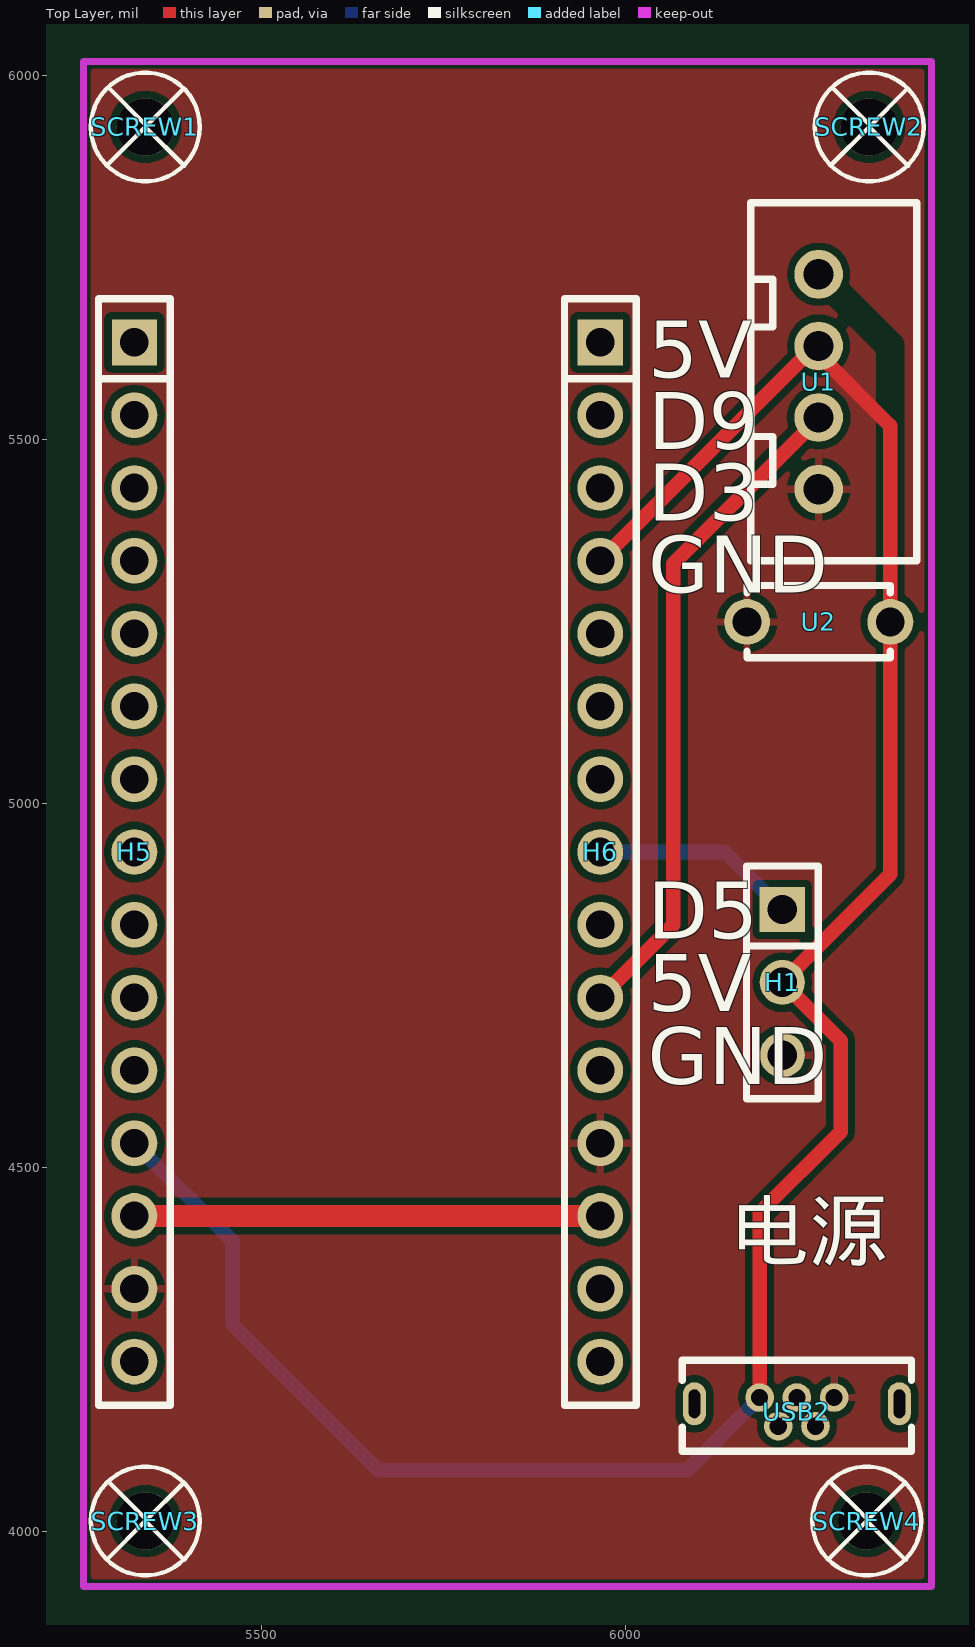
[diagram p0: Top Layer view]
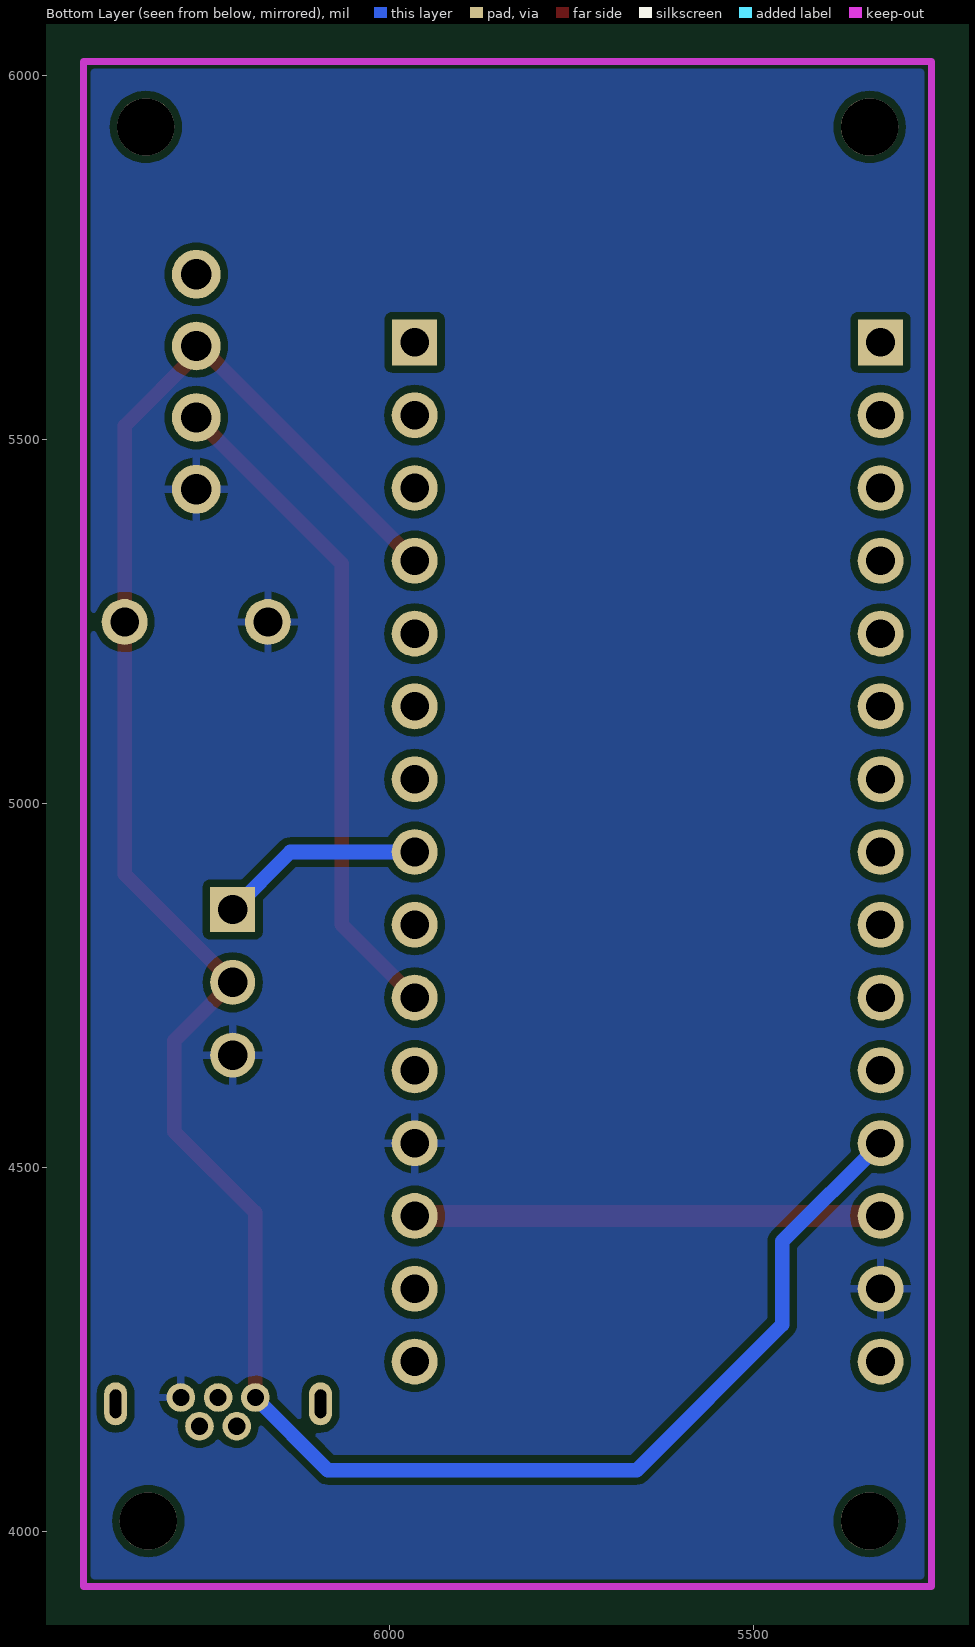
[diagram p1: Bottom Layer view, seen from below]
# Altium PCB MISC52018.pcbdoc
Units mil, origin at the board's own origin, x right, y up, seen from the top; angles counter-clockwise.
Board outline 5430 x 4915 mil, 2 copper layers (Top Layer, Bottom Layer), stack 62.206 mil thick; 10 components, 26 nets, 50 pads, 0 vias.

## Layer stack, top to bottom
Top Solder Mask Layer: solder mask 0.394, Dk 3.3
Top Layer: signal copper 1.379
Dielectric1: surface 59.449, FR4, Dk 4.5
Bottom Layer: signal copper 1.378
Bottom Solder Mask Layer: solder mask 0.394, Dk 3.3

## Board outline
8180,2750 2750,2750 2750,7665 8180,7665

## Design rules (kind name [scope] priority, off if disabled: settings)
BoardOutlineClearance copperThickness2oz_1 [All] p2 off: genericclearance=7.99 ignorepadtopadclearanceinfootprint=FALSE except(0: Arc-SplitContinuation Track-SplitContinuation SMDPad-SplitContinuation THPad-SplitContinuation Via-SplitContinuation Fill-SplitContinuation Region-SplitContinuation Poly-SplitContinuation Text-SplitContinuation Hole-SplitContinuation; 5.98: Arc-CutoutEdge Track-CutoutEdge SMDPad-CutoutEdge THPad-CutoutEdge Via-CutoutEdge Text-CutoutEdge; 6.9: Hole-OutlineEdge Hole-CutoutEdge; 10: Poly-OutlineEdge Poly-CutoutEdge; 11.81: Arc-OutlineEdge Track-OutlineEdge SMDPad-OutlineEdge THPad-OutlineEdge Via-OutlineEdge Fill-OutlineEdge Region-OutlineEdge Text-OutlineEdge Fill-CutoutEdge Region-CutoutEdge)
BoardOutlineClearance Plane_innerPlane_1 [All] p4 off: genericclearance=4.02 ignorepadtopadclearanceinfootprint=FALSE except(0: Arc-SplitContinuation Track-SplitContinuation SMDPad-SplitContinuation THPad-SplitContinuation Via-SplitContinuation Fill-SplitContinuation Region-SplitContinuation Poly-SplitContinuation Text-SplitContinuation Hole-SplitContinuation; 5.98: Arc-CutoutEdge Track-CutoutEdge SMDPad-CutoutEdge THPad-CutoutEdge Via-CutoutEdge Text-CutoutEdge; 6.9: Hole-OutlineEdge Hole-CutoutEdge; 10: Poly-OutlineEdge Poly-CutoutEdge; 11.81: Arc-OutlineEdge Track-OutlineEdge SMDPad-OutlineEdge THPad-OutlineEdge Via-OutlineEdge Fill-OutlineEdge Region-OutlineEdge Text-OutlineEdge Fill-CutoutEdge Region-CutoutEdge)
BoardOutlineClearance Copper_copperRegion_1 [All] p6 off: genericclearance=4.02 ignorepadtopadclearanceinfootprint=FALSE except(0: Arc-SplitContinuation Track-SplitContinuation SMDPad-SplitContinuation THPad-SplitContinuation Via-SplitContinuation Fill-SplitContinuation Region-SplitContinuation Poly-SplitContinuation Text-SplitContinuation Hole-SplitContinuation; 5.98: Arc-CutoutEdge Track-CutoutEdge SMDPad-CutoutEdge THPad-CutoutEdge Via-CutoutEdge Text-CutoutEdge; 6.9: Hole-OutlineEdge Hole-CutoutEdge; 10: Poly-OutlineEdge Poly-CutoutEdge; 11.81: Arc-OutlineEdge Track-OutlineEdge SMDPad-OutlineEdge THPad-OutlineEdge Via-OutlineEdge Fill-OutlineEdge Region-OutlineEdge Text-OutlineEdge Fill-CutoutEdge Region-CutoutEdge)
BoardOutlineClearance Copper_copperRegion_copperThickness1oz_1 [All] p8 off: genericclearance=4.02 ignorepadtopadclearanceinfootprint=FALSE except(0: Arc-SplitContinuation Track-SplitContinuation SMDPad-SplitContinuation THPad-SplitContinuation Via-SplitContinuation Fill-SplitContinuation Region-SplitContinuation Poly-SplitContinuation Text-SplitContinuation Hole-SplitContinuation; 5.98: Arc-CutoutEdge Track-CutoutEdge SMDPad-CutoutEdge THPad-CutoutEdge Via-CutoutEdge Text-CutoutEdge; 6.9: Hole-OutlineEdge Hole-CutoutEdge; 10: Poly-OutlineEdge Poly-CutoutEdge; 11.81: Arc-OutlineEdge Track-OutlineEdge SMDPad-OutlineEdge THPad-OutlineEdge Via-OutlineEdge Fill-OutlineEdge Region-OutlineEdge Text-OutlineEdge Fill-CutoutEdge Region-CutoutEdge)
BoardOutlineClearance Copper_copperRegion_Copper_copperRegion_1 [All] p10 off: genericclearance=4.02 ignorepadtopadclearanceinfootprint=FALSE except(0: Arc-SplitContinuation Track-SplitContinuation SMDPad-SplitContinuation THPad-SplitContinuation Via-SplitContinuation Fill-SplitContinuation Region-SplitContinuation Poly-SplitContinuation Text-SplitContinuation Hole-SplitContinuation; 5.98: Arc-CutoutEdge Track-CutoutEdge SMDPad-CutoutEdge THPad-CutoutEdge Via-CutoutEdge Text-CutoutEdge; 6.9: Hole-OutlineEdge Hole-CutoutEdge; 10: Poly-OutlineEdge Poly-CutoutEdge; 11.81: Arc-OutlineEdge Track-OutlineEdge SMDPad-OutlineEdge THPad-OutlineEdge Via-OutlineEdge Fill-OutlineEdge Region-OutlineEdge Text-OutlineEdge Fill-CutoutEdge Region-CutoutEdge)
BoardOutlineClearance copperThickness1oz_1 [All] p12: genericclearance=4.02 ignorepadtopadclearanceinfootprint=FALSE except(0: Arc-SplitContinuation Track-SplitContinuation SMDPad-SplitContinuation THPad-SplitContinuation Via-SplitContinuation Fill-SplitContinuation Region-SplitContinuation Poly-SplitContinuation Text-SplitContinuation Hole-SplitContinuation; 5.98: Arc-CutoutEdge Track-CutoutEdge SMDPad-CutoutEdge THPad-CutoutEdge Via-CutoutEdge Text-CutoutEdge; 6.9: Hole-OutlineEdge Hole-CutoutEdge; 10: Poly-OutlineEdge Poly-CutoutEdge; 11.81: Arc-OutlineEdge Track-OutlineEdge SMDPad-OutlineEdge THPad-OutlineEdge Via-OutlineEdge Fill-OutlineEdge Region-OutlineEdge Text-OutlineEdge Fill-CutoutEdge Region-CutoutEdge)
Clearance copperThickness2oz [All] p1 off: gap=7.99 ignorepadtopadclearanceinfootprint=FALSE except(5.98: SMDPad-Track SMDPad-SMDPad THPad-Track SMDPad-THPad THPad-THPad Track-Via SMDPad-Via THPad-Via Via-Via Fill-SMDPad Region-SMDPad Fill-THPad Region-THPad Fill-Via Region-Via Fill-Fill Fill-Region Region-Region Arc-Track Arc-SMDPad Arc-THPad Arc-Via Fill-Arc Region-Arc Arc-Arc Text-Track SMDPad-Text Text-THPad Text-Via Fill-Text Region-Text Arc-Text Text-Text; 6.9: Hole-Track Hole-SMDPad Hole-THPad Hole-Via Fill-Hole Region-Hole Hole-Arc Hole-Text; 10: Poly-Track Poly-SMDPad Poly-THPad Poly-Via Poly-Fill Poly-Region Poly-Poly Poly-Arc Poly-Text Poly-Hole; 11.81: Fill-Track Region-Track)
Clearance Plane_innerPlane [All] p3 off: gap=4.02 ignorepadtopadclearanceinfootprint=FALSE except(5.98: SMDPad-Track SMDPad-SMDPad THPad-Track SMDPad-THPad THPad-THPad Track-Via SMDPad-Via THPad-Via Via-Via Fill-SMDPad Region-SMDPad Fill-THPad Region-THPad Fill-Via Region-Via Fill-Fill Fill-Region Region-Region Arc-Track Arc-SMDPad Arc-THPad Arc-Via Fill-Arc Region-Arc Arc-Arc Text-Track SMDPad-Text Text-THPad Text-Via Fill-Text Region-Text Arc-Text Text-Text; 6.9: Hole-Track Hole-SMDPad Hole-THPad Hole-Via Fill-Hole Region-Hole Hole-Arc Hole-Text; 10: Poly-Track Poly-SMDPad Poly-THPad Poly-Via Poly-Fill Poly-Region Poly-Poly Poly-Arc Poly-Text Poly-Hole; 11.81: Fill-Track Region-Track)
Clearance Copper_copperRegion [All] p5 off: gap=4.02 ignorepadtopadclearanceinfootprint=FALSE except(5.98: SMDPad-Track SMDPad-SMDPad THPad-Track SMDPad-THPad THPad-THPad Track-Via SMDPad-Via THPad-Via Via-Via Fill-SMDPad Region-SMDPad Fill-THPad Region-THPad Fill-Via Region-Via Fill-Fill Fill-Region Region-Region Arc-Track Arc-SMDPad Arc-THPad Arc-Via Fill-Arc Region-Arc Arc-Arc Text-Track SMDPad-Text Text-THPad Text-Via Fill-Text Region-Text Arc-Text Text-Text; 6.9: Hole-Track Hole-SMDPad Hole-THPad Hole-Via Fill-Hole Region-Hole Hole-Arc Hole-Text; 10: Poly-Track Poly-SMDPad Poly-THPad Poly-Via Poly-Fill Poly-Region Poly-Poly Poly-Arc Poly-Text Poly-Hole; 11.81: Fill-Track Region-Track)
Clearance Copper_copperRegion_copperThickness1oz [All] p7 off: gap=4.02 ignorepadtopadclearanceinfootprint=FALSE except(5.98: SMDPad-Track SMDPad-SMDPad THPad-Track SMDPad-THPad THPad-THPad Track-Via SMDPad-Via THPad-Via Via-Via Fill-SMDPad Region-SMDPad Fill-THPad Region-THPad Fill-Via Region-Via Fill-Fill Fill-Region Region-Region Arc-Track Arc-SMDPad Arc-THPad Arc-Via Fill-Arc Region-Arc Arc-Arc Text-Track SMDPad-Text Text-THPad Text-Via Fill-Text Region-Text Arc-Text Text-Text; 6.9: Hole-Track Hole-SMDPad Hole-THPad Hole-Via Fill-Hole Region-Hole Hole-Arc Hole-Text; 10: Poly-Track Poly-SMDPad Poly-THPad Poly-Via Poly-Fill Poly-Region Poly-Poly Poly-Arc Poly-Text Poly-Hole; 11.81: Fill-Track Region-Track)
Clearance Copper_copperRegion_Copper_copperRegion [All] p9 off: gap=4.02 ignorepadtopadclearanceinfootprint=FALSE except(5.98: SMDPad-Track SMDPad-SMDPad THPad-Track SMDPad-THPad THPad-THPad Track-Via SMDPad-Via THPad-Via Via-Via Fill-SMDPad Region-SMDPad Fill-THPad Region-THPad Fill-Via Region-Via Fill-Fill Fill-Region Region-Region Arc-Track Arc-SMDPad Arc-THPad Arc-Via Fill-Arc Region-Arc Arc-Arc Text-Track SMDPad-Text Text-THPad Text-Via Fill-Text Region-Text Arc-Text Text-Text; 6.9: Hole-Track Hole-SMDPad Hole-THPad Hole-Via Fill-Hole Region-Hole Hole-Arc Hole-Text; 10: Poly-Track Poly-SMDPad Poly-THPad Poly-Via Poly-Fill Poly-Region Poly-Poly Poly-Arc Poly-Text Poly-Hole; 11.81: Fill-Track Region-Track)
Clearance copperThickness1oz [All] p11: gap=4.02 ignorepadtopadclearanceinfootprint=FALSE except(5.98: SMDPad-Track SMDPad-SMDPad THPad-Track SMDPad-THPad THPad-THPad Track-Via SMDPad-Via THPad-Via Via-Via Fill-SMDPad Region-SMDPad Fill-THPad Region-THPad Fill-Via Region-Via Fill-Fill Fill-Region Region-Region Arc-Track Arc-SMDPad Arc-THPad Arc-Via Fill-Arc Region-Arc Arc-Arc Text-Track SMDPad-Text Text-THPad Text-Via Fill-Text Region-Text Arc-Text Text-Text; 6.9: Hole-Track Hole-SMDPad Hole-THPad Hole-Via Fill-Hole Region-Hole Hole-Arc Hole-Text; 10: Poly-Track Poly-SMDPad Poly-THPad Poly-Via Poly-Fill Poly-Region Poly-Poly Poly-Arc Poly-Text Poly-Hole; 11.81: Fill-Track Region-Track)
DiffPairsRouting differentialPair [All] p1: maxlimit=6 minlimit=6 mostfreqgap=6 toplayer_minwidth=5 toplayer_prefwidth=10 toplayer_maxwidth=100 toplayer_mingap=6 toplayer_prefgap=6 toplayer_maxgap=6 bottomlayer_minwidth=5 bottomlayer_prefwidth=10 bottomlayer_maxwidth=100 bottomlayer_mingap=6 bottomlayer_prefgap=6 bottomlayer_maxgap=6 maxuncoupledlength=10
HoleToHoleClearance otherClearance [All] p1: gap=11.81 allowstackedmicrovias=TRUE
Length netLength [All] p1: minlimit=0 maxlimit=0
PasteMaskExpansion pasteMaskExpansion [All] p1: expansion=0
PlaneConnect innerPlane [All] p1: planeconnectstyle=Relief reliefexpansion=20 reliefentries=4 reliefconductorwidth=10 reliefairgap=10
PolygonConnect copperRegion_copperThickness1oz [All] p1 off: connectstyle=Relief reliefconductorwidth=10 reliefentries=4 polygonreliefangle="90 Angle" airgapwidth=10 via.connectstyle=Relief via.reliefconductorwidth=10 via.reliefentries=4 via.polygonreliefangle="90 Angle" via.airgapwidth=10
PolygonConnect copperRegion_Copper_copperRegion [All] p2 off: connectstyle=Relief reliefconductorwidth=10 reliefentries=4 polygonreliefangle="90 Angle" airgapwidth=10 via.connectstyle=Relief via.reliefconductorwidth=10 via.reliefentries=4 via.polygonreliefangle="90 Angle" via.airgapwidth=10
PolygonConnect copperRegion [All] p3: connectstyle=Relief reliefconductorwidth=10 reliefentries=4 polygonreliefangle="90 Angle" airgapwidth=10 via.connectstyle=Relief via.reliefconductorwidth=10 via.reliefentries=4 via.polygonreliefangle="90 Angle" via.airgapwidth=10
RoutingVias viaSize [All] p1: holewidth=12.01 width=24.02 viastyle="Through Hole" minholewidth=11.81 minwidth=19.68 maxholewidth=248.03 maxwidth=393.7
SolderMaskExpansion solderMaskExpansion [IsVia] p1: expansion=-1000 istentingtop=TRUE
SolderMaskExpansion solderMaskExpansion [All] p2: expansion=2 istentingtop=FALSE
Width copperThickness2oz_2 [All] p1 off: maxlimit=100 minlimit=8 preferedwidth=10
Width copperThickness1oz_2 [All] p2: maxlimit=100 minlimit=5 preferedwidth=10

## Components (designator, comment, footprint, x,y, rotation, side; value= is the part's Value field where it differs from the comment)
H1 "" HDR-TH_3P-P2.54-V-F 6215,4755 r270 top
H5 "" HDR-TH_15P-P2.54-V-F-1 5325,4934.06 r270 top
H6 "" HDR-TH_15P-P2.54-V-F-1 5965,4934.06 r270 top
SCREW1 "" M2螺丝 5340,5930 r0 top
SCREW2 "" M2螺丝 6334.36,5930 r0 top
SCREW3 "" M2螺丝 5340,4015 r0 top
SCREW4 "" M2螺丝 6330.91,4015 r0 top
U1 "XH2.54_4P_直插" CONN-TH_4P-P2.50-XH2.54-4P 6265,5580 r90 top
U2 "100nF" CAP-TH_L5.0-W2.5-P5.00-D1.0 6265,5250 r180 top
USB2 "HXMICRO180JB2" MICRO-USB-TH_HXMICRO180JB2 6235,4165 r0 top

## Footprints (in the part's own frame and the unit in brackets; to place one, negate y for a bottom-side part, rotate by r counter-clockwise, add the part's x,y. Pads: shape width x height; smd on the part's side, far side on the other; paste and mask are expansions set on the pad)
CAP-TH_L5.0-W2.5-P5.00-D1.0 [mm]
  round 1.6 hole 1: 1(-2.5,0) 2(2.5,0)
  silkscreen extent -2.5,-1.27 2.5,1.25
CONN-TH_4P-P2.50-XH2.54-4P [mm]
  round 1.7 hole 1.05 paste+0 mask+0.05: 1(3.75,0) 2(1.25,0) 3(-1.25,0) 4(-3.75,0)
  silkscreen extent -6.25,-3.42 6.25,2.37
HDR-TH_3P-P2.54-V-F [mil]
  rect 62x62 hole 40.16: 1(-100,0)
  round 62 hole 40.16: 2(0,0) 3(100,0)
  silkscreen extent -160,-49 160,49
HDR-TH_15P-P2.54-V-F-1 [mm]
  rect 1.6x1.575 hole 1: 1(-17.78,0)
  round 1.6 hole 1: 2(-15.24,0) 3(-12.7,0) 4(-10.16,0) 5(-7.62,0) 6(-5.08,0) 7(-2.54,0) 8(0,0) 9(2.54,0) 10(5.08,0) 11(7.62,0) 12(10.16,0) 13(12.7,0) 14(15.24,0) 15(17.78,0)
  silkscreen extent -19.3,-1.25 19.3,1.25
M2螺丝 [mm]
  round 2 hole 2: 1(0,0)
  silkscreen extent -1.9,-1.9 1.9,1.9
MICRO-USB-TH_HXMICRO180JB2 [mm]
  round 1 hole 0.6: 1(-1.3,0.5) 2(-0.65,-0.5) 3(0,0.5) 4(0.65,-0.5) 5(1.3,0.5)
  oval 0.8x1.5 hole 0.4 slot 1 at 90 deg: 6(3.575,0.28) 7(-3.575,0.28)
  silkscreen extent -4,-1.37 4,1.8

## Nets (pads, with @x,y where several pads share a name; then routed paths per layer and width w, separated by ;. In a path a pad name is that pad's centre, name@x,y a point inside that pad or via, vN(x,y) a via of type N, cw(c..) or ccw(c..) an arc to the next point about the centre after c; other vN are vias at no path point)
+5V: H1.2 H5.12 U1.1 U2.1 USB2.1 | length 2877.3
  Top Layer w20: USB2.1 6183.82,4438.82 6295,4550 6295,4675 H1.2 6363.43,4903.43 U2.1 ; 6265,5617.64 6363.43,5519.21 6363.43,5140
  Bottom Layer w20: H5.12 5460,4399.06 5460,4285 5660,4085 6084.14,4085 USB2.1
A0: H5.4
A1: H5.5
A2: H5.6
A3: H5.7
A4: H5.8
A5: H5.9
A6: H5.10
A7: H5.11
D2: H6.11
D3: H6.10 U1.3 | length 921
  Top Layer w20: H6.10 6065,4834.06 6065,5330 6265,5530 U1.3
D4: H6.9
D5: H1.1 H6.8 | length 282.7
  Bottom Layer w20: H6.8 6135.94,4934.06 H1.1
D6: H6.7
D7: H6.6
D8: H6.5
D9: H6.4 U1.2 | length 422.3
  Top Layer w20: H6.4 6260.16,5629.21 U1.2
D10: H6.3
D11: H6.2
D12: H6.1
D13: H5.1
GND: H1.3 H5.14 H6.12 U1.4 U2.2 USB2.5
REF: H5.3
RST: H5.13 H6.13 | length 640
  Top Layer w30: H5.13 H6.13
RXD: H6.14
TXD: H6.15
pads on no net: H5.2 H5.15 SCREW1.1 SCREW2.1 SCREW3.1 SCREW4.1 USB2.2 USB2.3 USB2.4 USB2.6 USB2.7

## Polygon pours and split planes (outlines as drawn)
GND on Bottom Layer (solid, remove dead copper, pour order 2): 3525,7245 3525,3080 7700,3080 7700,7245
GND on Top Layer (solid, remove dead copper, pour order 2): 3000,7415 3000,3000 7930,3000 7930,7415

## Keep-outs
Board Outline Layer:
  lines w10: 5255,3925 5255,6020 6420,6020 6420,3925 5255,3925

## Silkscreen, mask and mechanical layers (free items; w line width, h text height)
Top Silkscreen Layer:
  text "5V" at 6030.63,5585.63 h78.74
  text "D9" at 6030.63,5487.2 h78.74
  text "D3" at 6030.63,5388.78 h78.74
  text "GND" at 6030.63,5290.35 h78.74
  text "D5" at 6030,4815 h78.74
  text "5V" at 6030,4715 h78.74
  text "GND" at 6030,4615 h78.74
  text "电源" at 6145,4375 h78.74